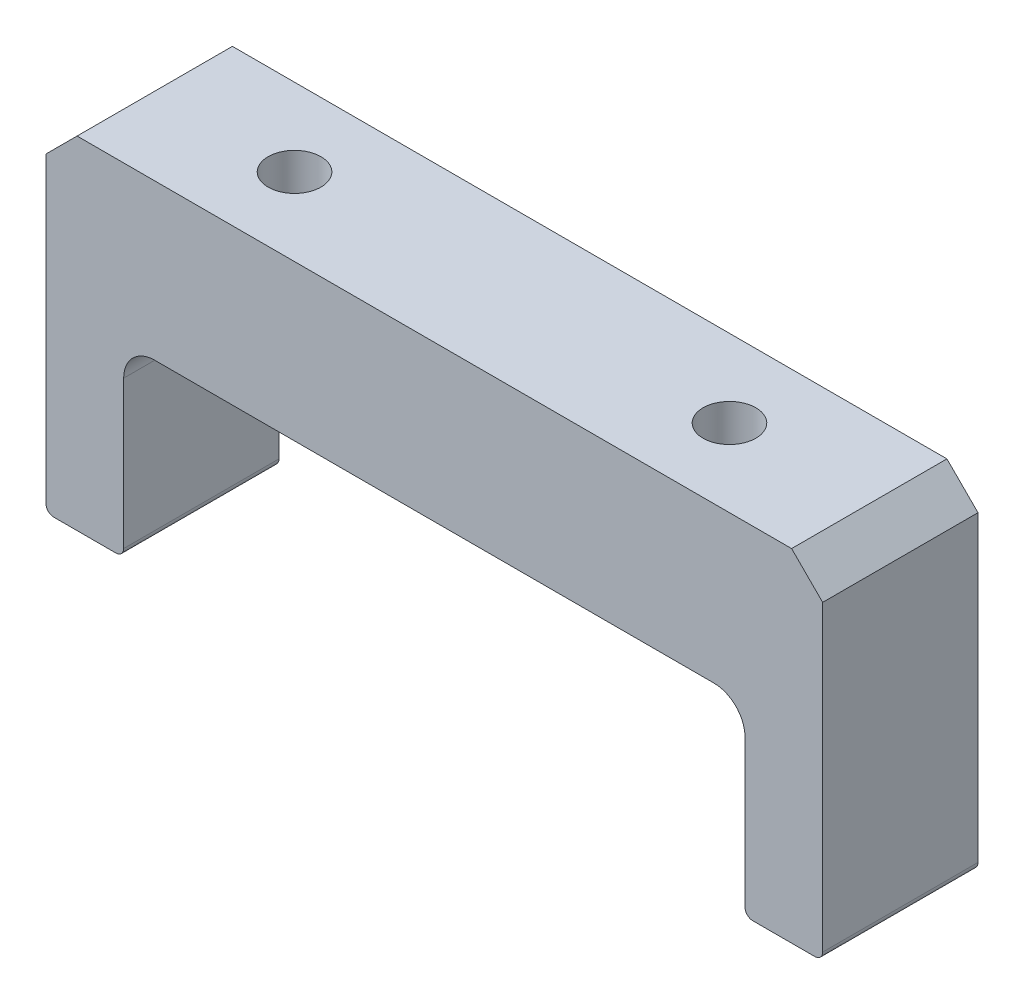
SolidWorks part; units mm, degrees
material "S45C"
ref_plane "Front Plane" through (0, 0, 0) normal (0, 0, 1) x (1, 0, 0)
ref_plane "Top Plane" through (0, 0, 0) normal (0, 1, 0) x (1, 0, 0)
ref_plane "Right Plane" through (0, 0, 0) normal (1, 0, 0) x (0, 0, -1)
sketch "Sketch1" plane through (0, 0, 0) normal (0, 0, 1) x (1, 0, 0)
  line L0 (45, -22) -> (50, -22)
  line L1 (0, 0) -> (50, 0)
  line L2 (0, 0) -> (0, -22)
  line L3 (0, -22) -> (5, -22)
  line L4 (50, 0) -> (50, -22)
  line L6 (5, -22) -> (5, -10)
  line L7 (5, -10) -> (45, -10)
  line L8 (45, -22) -> (45, -10)
  dimension "D1" = 5
  dimension "D2" = 5
  dimension "D3" = 12
  dimension "D4" = 10
  dimension "D5" = 40
extrude "Boss-Extrude1" add sketch "Sketch1" along normal blind 10
hole_wizard "CBORE for M3 Hex Head Bolt1" positions "Sketch3" profile "Sketch2" counterbore size "M3" standard "GB" end condition through all
sketch "Sketch3" plane through (0, -10, 0) normal (0, -1, 0) x (1, 0, 0)
  line L0 (25, 10) -> (25, 0) construction
  line L1 (5, 10) -> (45, 10) construction
  line L2 (5, 0) -> (45, 0) construction
  line L4 (25, 5) -> (11, 5) construction
  point P0 (11, 5)
  point P1 (39, 5)
  dimension "D1" = 28
sketch "Sketch2" plane through (11, -10, 5) normal (1, 0, 0) x (0, 0, -1)
  line L0 (0, 0) -> (0, 10)
  line L1 (0, 10) -> (1.7, 10)
  line L3 (1.7, 10) -> (1.7, 3.5)
  line L4 (1.7, 3.5) -> (3, 3.5)
  line L5 (3, 3.5) -> (3, 0)
  line L7 (3, 0) -> (0, 0)
  line L11 (0, -6.35) -> (0, 107.95) construction
  dimension "通孔孔直径" = 3.4
  dimension "通孔孔深度" = 10
  dimension "柱形沉头孔直径" = 6
  dimension "柱形沉头孔深度" = 3.5
fillet "Fillet1" radius 2 2 edges at (45, -10, 5) (5, -10, 5)
fillet "Fillet2" radius 0.5 4 edges at (50, -22, 5) (45, -22, 5) (5, -22, 5) (0, -22, 5)
chamfer "Chamfer1" distance 2 angle 45 2 edges at (50, 0, 5) (0, 0, 5)
